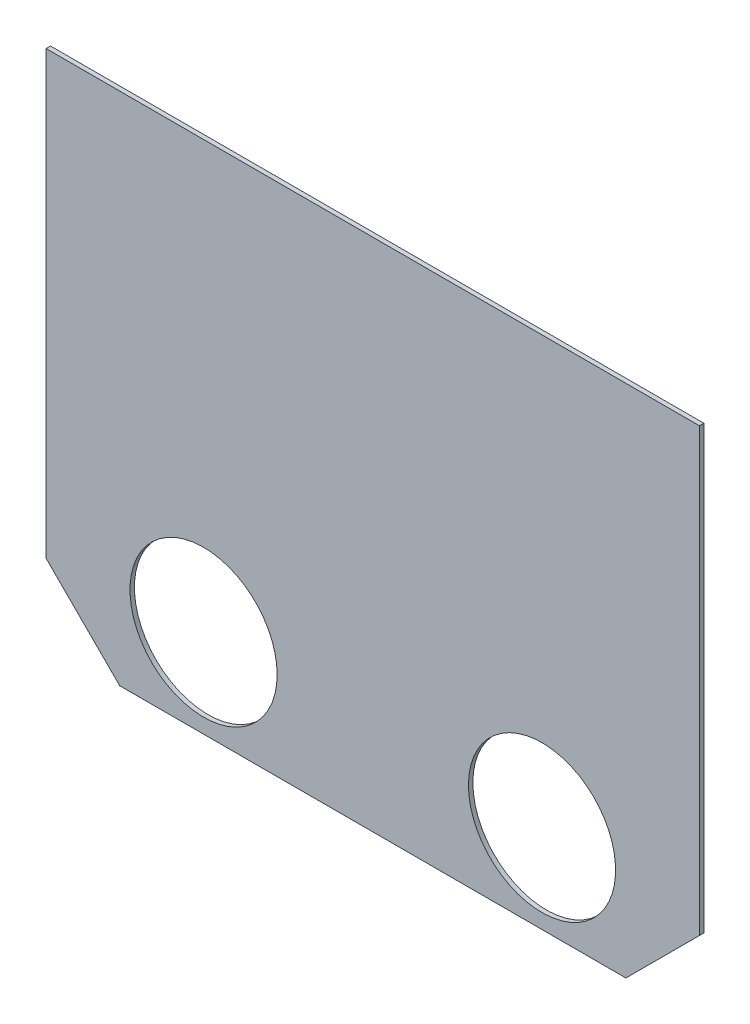
from build123d import *

# Parameters (mm, degrees)
SKETCH1_R           = 50
BOSS_EXTRUDE1_DEPTH = 1.5


with BuildPart() as part:
    # Sketch1 → Boss-Extrude1 (new, symmetric)
    with BuildSketch(Plane.XY):
        Polygon((50, 0), (394, 0), (444, 50), (444, 350), (0, 350), (0, 50), align=None)
        with Locations((107, 60)):
            Circle(SKETCH1_R, mode=Mode.SUBTRACT)
        with Locations(Location((337, 60, 0), (0, 0, 180))):
            Circle(SKETCH1_R, mode=Mode.SUBTRACT)
    extrude(amount=BOSS_EXTRUDE1_DEPTH, both=True)


solid = part.part
